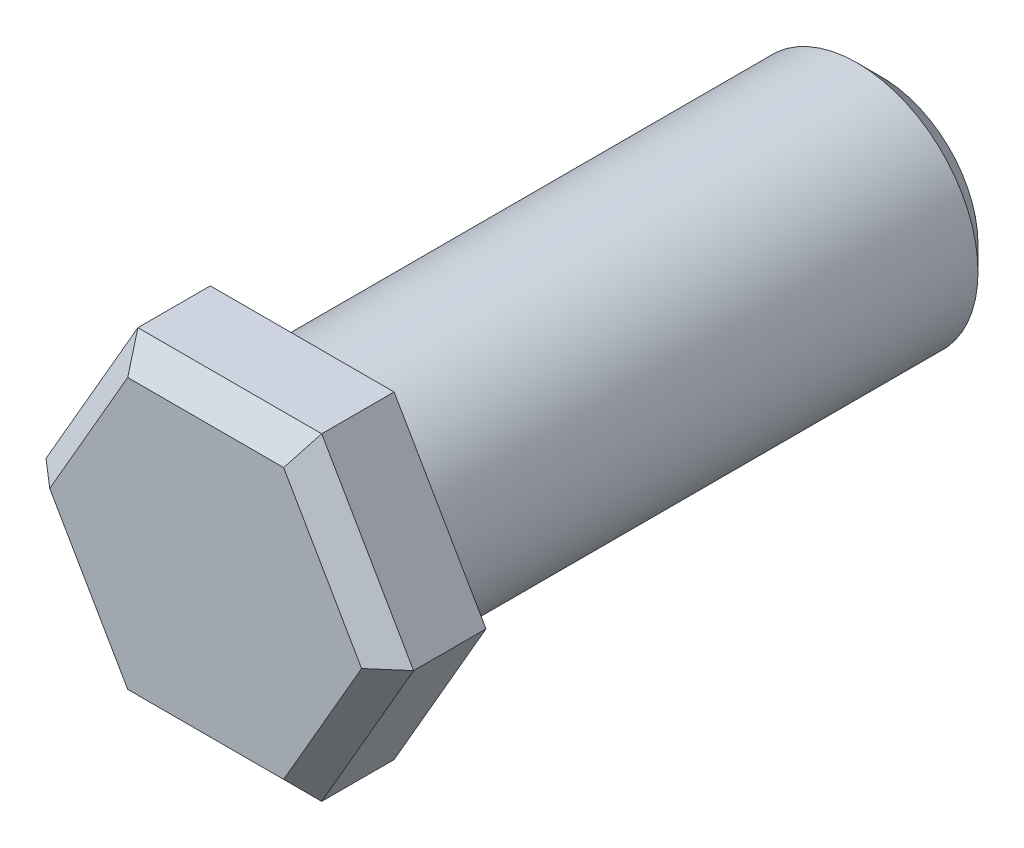
from build123d import *

# Parameters (mm, degrees)
SKETCH1_R           = 2.5
BOSS_EXTRUDE1_DEPTH = 12
BOSS_EXTRUDE2_DEPTH = 2
CHAMFER1_SIZE       = 0.5


with BuildPart() as part:
    # Sketch1 → Boss-Extrude1 (new body)
    with BuildSketch(Plane.XY):
        with Locations((720, 45)):
            Circle(SKETCH1_R)
    extrude(amount=-BOSS_EXTRUDE1_DEPTH)

    # Sketch2 → Boss-Extrude2 (add)
    with BuildSketch(Plane.XY):
        Polygon((718.096078213, 41.702310731), (721.903921787, 41.702310731), (723.807843574, 45), (721.903921787, 48.297689269), (718.096078213, 48.297689269), (716.192156426, 45), align=None)
    extrude(amount=BOSS_EXTRUDE2_DEPTH)

    # Chamfer1
    chamfer1_edges = [part.edges().sort_by_distance(p)[0] for p in [
        (717.5, 45, -12),
        (717.144117319, 43.351155365, 2),
        (720, 41.702310731, 2),
        (722.855882681, 43.351155365, 2),
        (722.855882681, 46.648844635, 2),
        (720, 48.297689269, 2),
        (717.144117319, 46.648844635, 2),
    ]]
    chamfer(chamfer1_edges, length=CHAMFER1_SIZE)


solid = part.part
